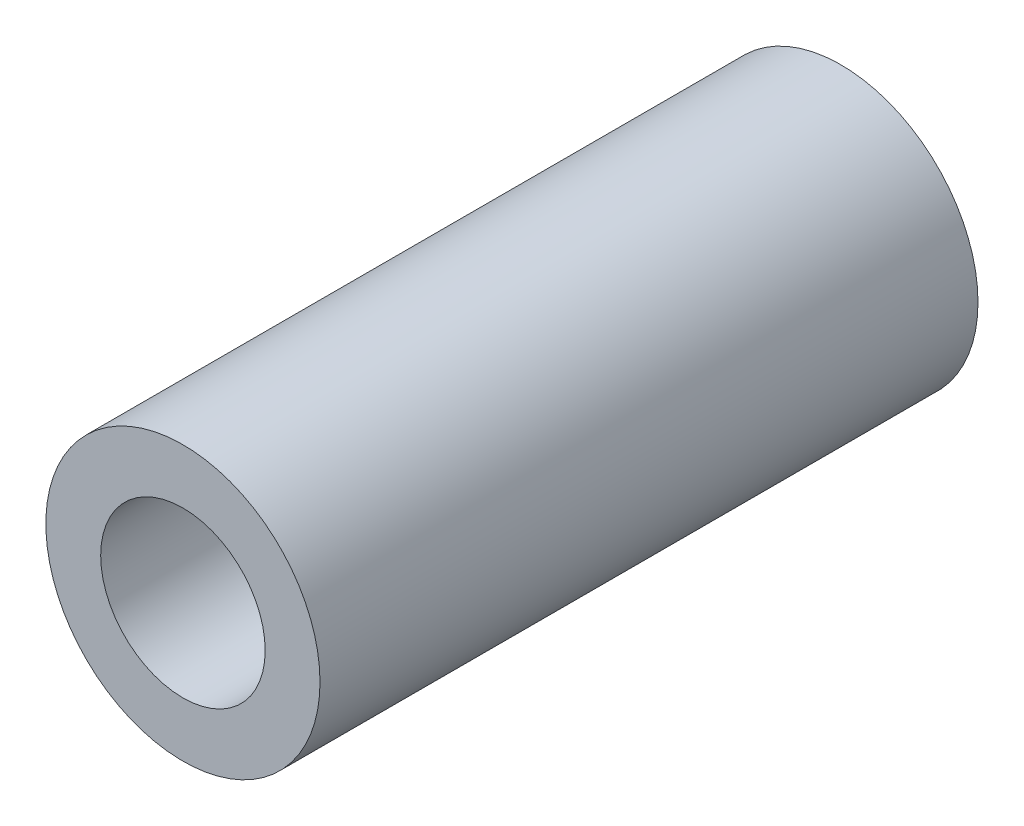
SolidWorks part; units mm, degrees
material "Plain Carbon Steel"
ref_plane "Front Plane" through (0, 0, 0) normal (0, 0, 1) x (1, 0, 0)
ref_plane "Top Plane" through (0, 0, 0) normal (0, 1, 0) x (1, 0, 0)
ref_plane "Right Plane" through (0, 0, 0) normal (1, 0, 0) x (0, 0, -1)
sketch "Sketch1" plane through (0, 0, 0) normal (0, 0, 1) x (1, 0, 0)
  circle A0 centre (0, 0) radius 6
  circle A1 centre (0, 0) radius 10
  dimension "D1" = 12
  dimension "D2" = 20
extrude "Boss-Extrude1" add sketch "Sketch1" along normal blind 48
